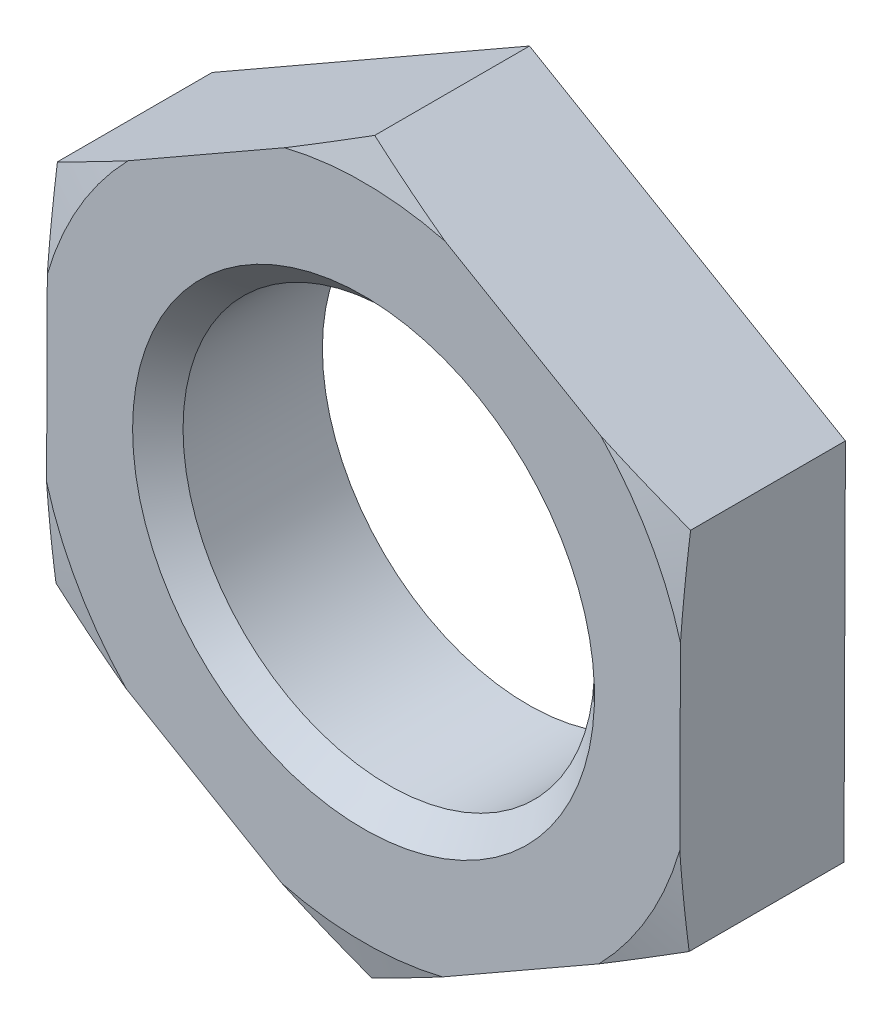
SolidWorks part; units mm, degrees
extrude "基体-拉伸" add sketch "草图1" along normal blind 8.4
sketch "草图1" plane through (0, 0, 0) normal (0, 0, 1) x (1, 0, 0)
  line L0 (-26.8088, 0) -> (37.1748, 0) construction
  line L1 (0, 25.0215) -> (0, -25.0215) construction
  line L3 (0.035, 8.8849) -> (-7.6771, 4.4727)
  line L4 (-7.6771, 4.4727) -> (-7.7121, -4.4122)
  line L5 (-7.7121, -4.4122) -> (-0.035, -8.8849)
  line L6 (-0.035, -8.8849) -> (7.6771, -4.4727)
  line L7 (7.6771, -4.4727) -> (7.7121, 4.4122)
  line L8 (7.7121, 4.4122) -> (0.035, 8.8849)
  circle A0 centre (0, 0) radius 7.6946 construction
  circle A1 centre (0, 0) radius 5
cosmetic thread "装饰螺纹线1"
chamfer "倒角1" distance 0.6131 angle 45 2 edges at (5, 0, 0) (5, 0, 8.4)
material "A2-70级"
ref_plane "基准面1" through (0, 0, 0) normal (0, 0, 1) x (1, 0, 0)
ref_plane "基准面2" through (0, 0, 0) normal (0, 1, 0) x (1, 0, 0)
ref_plane "基准面3" through (0, 0, 0) normal (1, 0, 0) x (0, 0, -1)
sketch "尺寸草图" plane through (0, 0, 0) normal (0, 0, 1) x (1, 0, 0)
  line L0 (0, 0) -> (26.6749, 0)
  line L1 (26.6749, 0) -> (37.4249, 0)
  line L2 (37.4249, 0) -> (52.0249, 0)
  line L3 (-9.5238, 0) -> (0, 0)
  point P3 (10, 0)
  point P4 (1.5, 0)
  point P5 (17.77, 0)
  point P6 (8.4, 0)
  point P7 (6.4, 0)
  point P8 (16, 0)
sketch "草图2" plane through (0, 0, 0) normal (0, 0, -1) x (-1, 0, 0)
  circle A0 centre (0, 0) radius 8
  circle A1 centre (0, 0) radius 5 construction
extrude "切除-拉伸1" cut sketch "草图2" against normal through all draft 75 flip side to cut
sketch "草图3" plane through (0, 0, 8.4) normal (0, 0, 1) x (1, 0, 0)
  circle A0 centre (0, 0) radius 8
extrude "切除-拉伸2" cut sketch "草图3" against normal through all draft 75 flip side to cut
sketch "草图4" plane through (0, 0, 0) normal (0, 0, -1) x (-1, 0, 0)
  circle A0 centre (0, 0) radius 10
  dimension "D1" = 20
extrude "切除-拉伸3" cut sketch "草图4" against normal blind 4.4
equation "\"e@草图1\" = \"e@尺寸草图\""
equation "\"D1@尺寸草图\" = \"D@尺寸草图\" / 1.05"
equation "\"D@草图1\" = \"D@尺寸草图\""
equation "\"m@基体-拉伸\" = \"m@尺寸草图\""
equation "\"D1@草图3\" = \"s@尺寸草图\""
equation "\"s@草图2\" = \"s@尺寸草图\""
equation "\"D2@装饰螺纹线1\" =\"D@尺寸草图\""
equation "\"D1@倒角1\" =  ( \"da@尺寸草图\" - \"D1@尺寸草图\" )  / 2"
